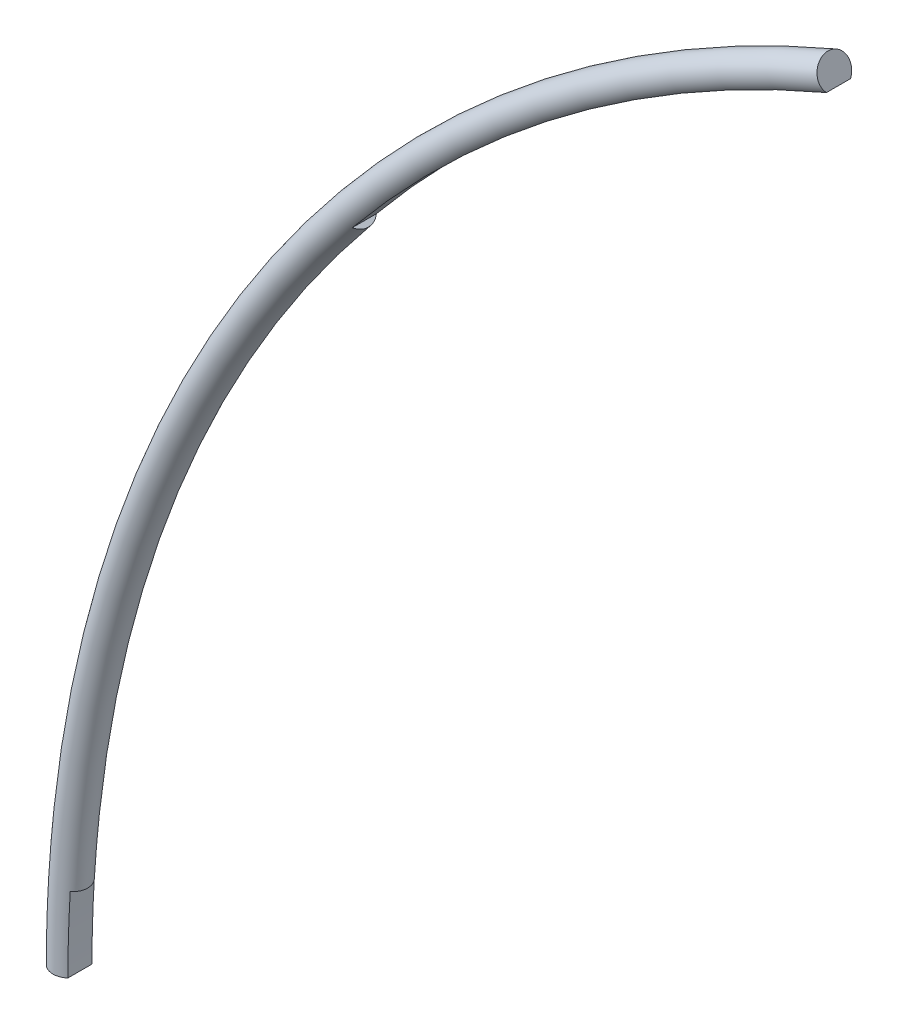
SolidWorks part; units mm, degrees
ref_plane "Front Plane" through (0, 0, 0) normal (0, 0, 1) x (1, 0, 0)
ref_plane "Top Plane" through (0, 0, 0) normal (0, 1, 0) x (1, 0, 0)
ref_plane "Right Plane" through (0, 0, 0) normal (1, 0, 0) x (0, 0, -1)
sketch "Sketch1" plane through (0, 0, 0) normal (0, 0, 1) x (1, 0, 0)
  line L0 (0, 0) -> (-121.3358, 0) construction
  line L1 (0, 0) -> (-43.6654, 102.8692) construction
  arc A0 (-91.0404, 214.4776) -> (-233, 0) centre (0, 0) ccw
  dimension "D1" = 67
  dimension "D2" = 233
sweep "Sweep1" add path "Sketch1" circular profile diameter 6 parameters "D3"=6
sketch "Sketch6" plane through (0, 0, 0) normal (0, 0, 1) x (1, 0, 0)
  line L0 (0, 0) -> (-231, 0)
  line L1 (0, 0) -> (-230.5691, 14.1022)
  line L2 (0, 0) -> (-178.2453, 146.9341)
  line L3 (0, 0) -> (-90.2589, 212.6366)
  line L4 (-89.8682, 211.7161) -> (-92.2125, 217.2391) construction
  arc A0 (-90.2589, 212.6366) -> (-178.2453, 146.9341) centre (0, 0) ccw
  arc A1 (-230.5691, 14.1022) -> (-231, 0) centre (0, 0) ccw
  dimension "D1" = 462
  dimension "D2" = 3.5
  dimension "D3" = 36
extrude "Cut-Extrude1" cut sketch "Sketch6" against normal mid plane 50 contours L1 A1 L0 | L3 A0 L2
